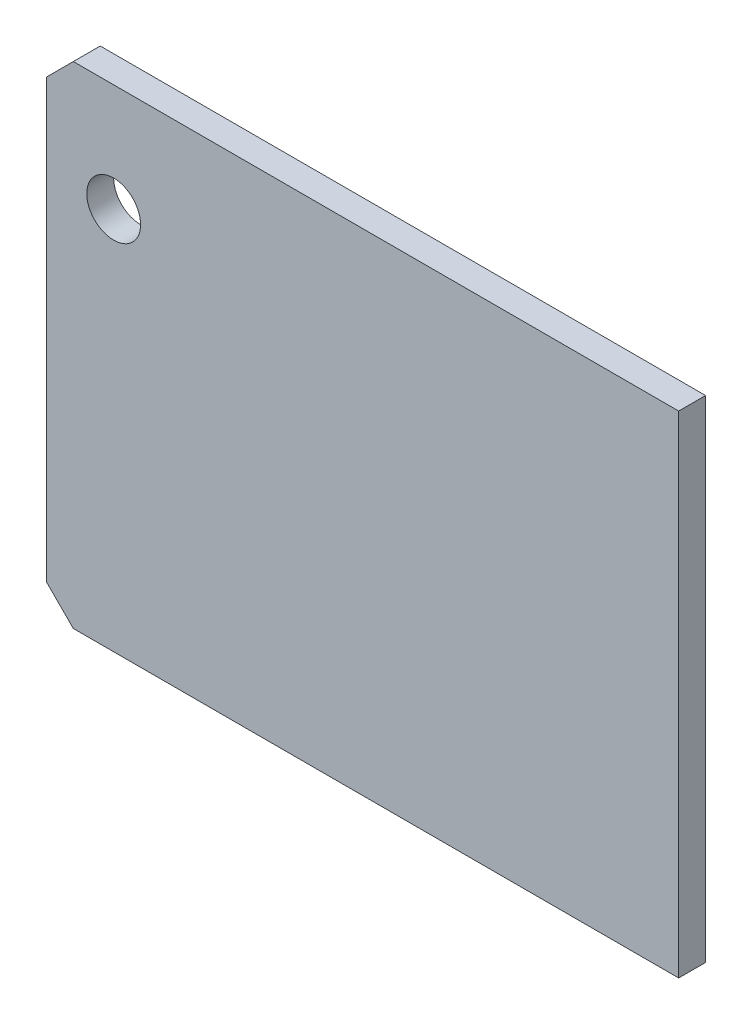
from build123d import *

# Parameters (mm, degrees)
SKETCH1_W               = 470
SKETCH1_H               = 365
BOSS_EXTRUDE1_DEPTH     = 20
CHAMFER1_SIZE           = 20
CUT_EXTRUDE1_DEPTH      = 299.213430281
CUT_EXTRUDE1_DEPTH_BACK = 299.213430281
SKETCH2_R               = 20
CHAMFER2_SIZE           = 20


with BuildPart() as part:
    # Sketch1 → Boss-Extrude1 (new body)
    with BuildSketch(Plane.XY):
        Rectangle(SKETCH1_W, SKETCH1_H)
    extrude(amount=BOSS_EXTRUDE1_DEPTH)

    # Chamfer1
    chamfer1_edges = [part.edges().sort_by_distance(p)[0] for p in [
        (-235, 182.5, 10),
    ]]
    chamfer(chamfer1_edges, length=CHAMFER1_SIZE)

    # Sketch2 → Cut-Extrude1 (cut, two sides: drawn at the far end of the back side and taken through both)
    with BuildSketch(Plane.XY.offset(20).offset(-CUT_EXTRUDE1_DEPTH_BACK)):
        with Locations((-185, 102.5)):
            Circle(SKETCH2_R)
    extrude(amount=CUT_EXTRUDE1_DEPTH + CUT_EXTRUDE1_DEPTH_BACK, mode=Mode.SUBTRACT)

    # Chamfer2
    chamfer2_edges = [part.edges().sort_by_distance(p)[0] for p in [
        (-235, -182.5, 10),
    ]]
    chamfer(chamfer2_edges, length=CHAMFER2_SIZE)


solid = part.part
